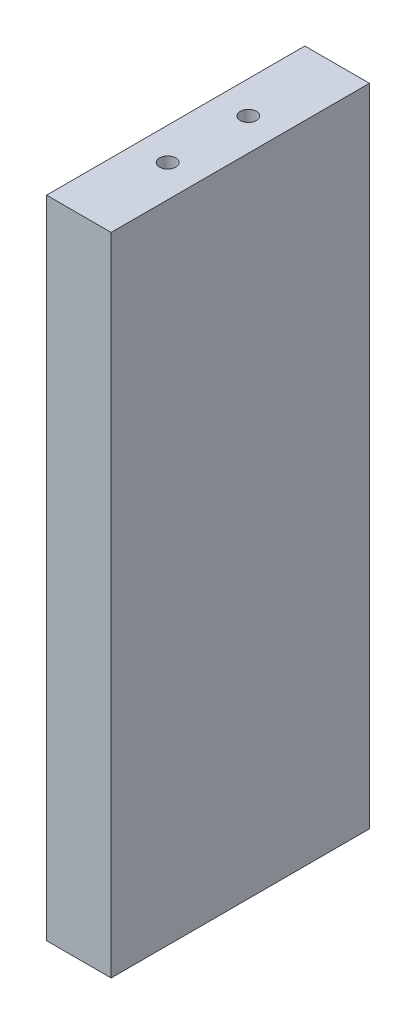
from build123d import *

# Parameters (mm, degrees)
SKETCH_1_W             = 80
SKETCH_1_H             = 200
EXTRUDE_1_DEPTH        = 20
HOLE_WIZARD_M6_1_D     = 5
HOLE_WIZARD_M6_1_DEPTH = 20
HOLE_WIZARD_M6_1_TIP   = 1.502151548
HOLE_WIZARD_M6_2_D     = 5
HOLE_WIZARD_M6_2_DEPTH = 23
HOLE_WIZARD_M6_2_TIP   = 1.502151548


with BuildPart() as part:
    # 草图1 → 凸台-拉伸1 (new body)
    with BuildSketch(Plane(origin=(0, 0, 0), x_dir=(0, 0, -1), z_dir=(1, 0, 0))):
        Rectangle(SKETCH_1_W, SKETCH_1_H)
    extrude(amount=EXTRUDE_1_DEPTH)

    # M6 螺纹孔1
    with Locations(Plane(origin=(0, 100, 0), x_dir=(1, 0, 0), z_dir=(0, 1, 0))):
        with Locations((10, 12.5), (10, -12.5)):
            Hole(HOLE_WIZARD_M6_1_D / 2, depth=HOLE_WIZARD_M6_1_DEPTH)
            with Locations((0, 0, -(HOLE_WIZARD_M6_1_DEPTH + HOLE_WIZARD_M6_1_TIP / 2))):  # 118° drill point
                Cone(0, HOLE_WIZARD_M6_1_D / 2, HOLE_WIZARD_M6_1_TIP, mode=Mode.SUBTRACT)

    # M6 螺纹孔2
    with Locations(Plane(origin=(0, -100, 0), x_dir=(-1, 0, 0), z_dir=(0, -1, 0))):
        with Locations((-10, 20), (-10, -20)):
            Hole(HOLE_WIZARD_M6_2_D / 2, depth=HOLE_WIZARD_M6_2_DEPTH)
            with Locations((0, 0, -(HOLE_WIZARD_M6_2_DEPTH + HOLE_WIZARD_M6_2_TIP / 2))):  # 118° drill point
                Cone(0, HOLE_WIZARD_M6_2_D / 2, HOLE_WIZARD_M6_2_TIP, mode=Mode.SUBTRACT)


solid = part.part
